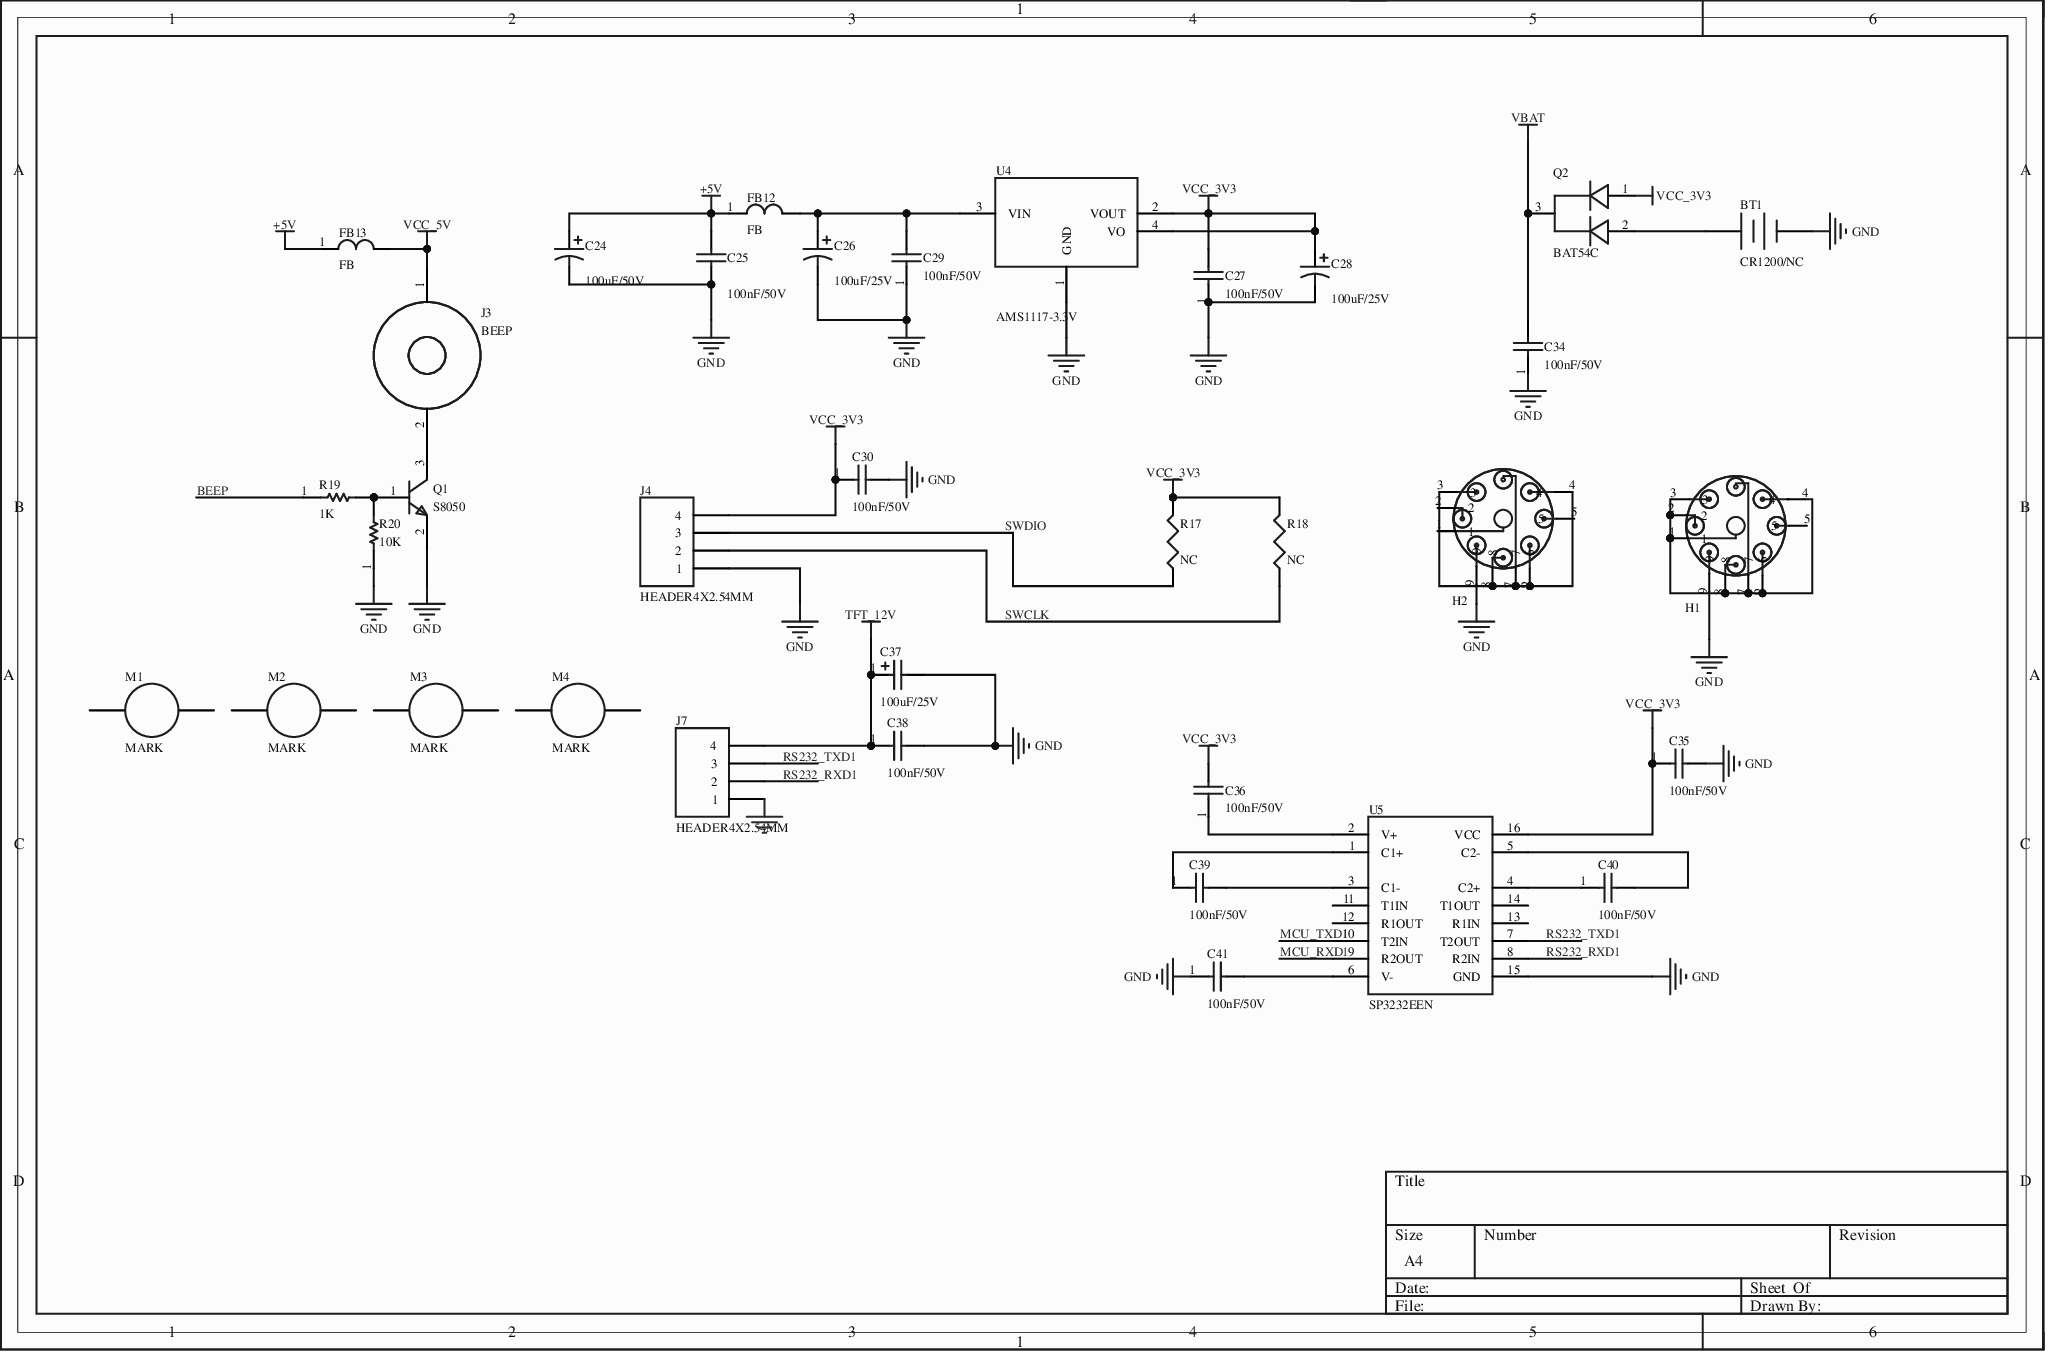
[diagram p0: MISC49890-3.schdoc]
# Altium project MISC49890-2.PrjPcb
1 sheet, 35 parts. Net scope: global (net labels, ports and power ports of the same name join across sheets).
Board file: MISC49890.pcbdoc

## Sheet MISC49890-3.schdoc
size 292 x 193 mm; @Page No: 1; @Page Count: 1; @Schematic Name: MISC49890; @Project Name: MISC49890; @Board Name: MISC49890; @Update Date: 2024-12-12; @Create Time: 18:15:27; @Update Time: 18:15:33; @Create Date: 2024-12-12

### Parts
BT1  CR1200/NC  [BAT-2]
C24  value 100uF/50V  [C0805]
C25  value 100nF/50V  [RAD-0.3]
C26  value 100uF/25V  [C0805]
C27  value 100nF/50V  [0603_C]  (hidden comment: Cap)
C28  value 100uF/25V  [C0805]
C29  value 100nF/50V  [0603_C]  (hidden comment: Cap)
C30  value 100nF/50V  [0603_C]  (hidden comment: Cap)
C34  value 100nF/50V  [0603_C]  (hidden comment: Cap)
C35  value 100nF/50V  [0603_C]  (hidden comment: Cap)
C36  value 100nF/50V  [0603_C]  (hidden comment: Cap)
C37  value 100uF/25V  [CAP-SMD_BD6.3-L6.6-W6.6-FD]  (hidden comment: Cap Pol1)
C38  value 100nF/50V  [0603_C]  (hidden comment: Cap)
C39  value 100nF/50V  [0603_C]  (hidden comment: Cap)
C40  value 100nF/50V  [0603_C]  (hidden comment: Cap)
C41  value 100nF/50V  [0603_C]  (hidden comment: Cap)
FB12  FB  [0603_L]
FB13  FB  [0603_L]
H1  H  [HOLE-ZR]  (value not drawn)
H2  H  [HOLE-ZR]  (value not drawn)
J3  BEEP  [BUZ-TH_BD12.0-P7.60-D0.6-FD]
J4  HEADER4X2.54MM  [CN4$2F$DIP$2F$P2.54B]
J7  HEADER4X2.54MM  [CN4$2F$DIP$2F$P2.54B]
M1  MARK  [RAD-0.1]
M2  MARK  [RAD-0.1]
M3  MARK  [RAD-0.1]
M4  MARK  [RAD-0.1]
Q1  S8050  [SOT-23(SOT-23-3)]
Q2  BAT54C  [SOT-23(SOT-23-3)]
R17  value NC  [J1-0603]
R18  value NC  [J1-0603]
R19  1K  [0603_R]
R20  10K  [0603_R]
U4  AMS1117-3.3V  [SOT-223]
U5  SP3232EEN  [SOP-16_150MIL]

### Nets
+5V: C24.1 C25.2 FB12.1 FB13.1
GND: BT1.2(-) C24.2 C25.1 C26.2 C27.1 C28.2 C29.1 C30.2 C34.1 C35.2 C37.2 C38.2 C41.1 H1.9 H2.9 J4.1 J7.1 Q1.2(E) R20.1 U4.1(GND) U5.15(GND)
TFT_12V: C37.1 C38.1 J7.4
VBAT: C34.2 Q2.3(K)
VCC_3V3: C27.2 C28.1 C30.1 C35.1 C36.2 J4.4 Q2.1(A1) R17.2 R18.2 U4.2(VOUT) U4.4(VO) U5.16(VCC)
VCC_5V: FB13.2 J3.1
BEEP: R19.1
MCU_RXD1: U5.9(R2OUT)
MCU_TXD1: U5.10(T2IN)
RS232_RXD1: J7.2 U5.8(R2IN)
RS232_TXD1: J7.3 U5.7(T2OUT)
SWCLK: J4.2 R18.1
SWDIO: J4.3 R17.1
NetBT1_1: BT1.1(+) Q2.2(A2)
NetC26_1: C26.1 C29.2 FB12.2 U4.3(VIN)
NetC36_1: C36.1 U5.2(V+)
NetC39_1: C39.1 U5.1(C1+)
NetC39_2: C39.2 U5.3(C1-)
NetC40_1: C40.1 U5.4(C2+)
NetC40_2: C40.2 U5.5(C2-)
NetC41_2: C41.2 U5.6(V-)
NetH1_1: H1.1 H1.2 H1.3 H1.4 H1.6 H1.7 H1.8
NetH2_3: H2.3 H2.4 H2.6 H2.7 H2.8
NetJ3_2: J3.2 Q1.3(C)
NetQ1_1: Q1.1(B) R19.2 R20.2

Not connected (* = marked no-connect by the designer): H1 5; H2 1 2 5; M1 1 2; M2 1 2; M3 1 2; M4 1 2; U5 11(T1IN)* 12(R1OUT)* 13(R1IN)* 14(T1OUT)*

### Notes on the sheet
- 1
- 2
- 3
- 4
- 5
- 6
- A
- B
- C
- D
- Title
- File:
- Date:
- Size
- A4
- Number
- Drawn By:
- Sheet
- Of
- Revision

### Library data of the parts
BT1 = CR1200/NC: Multicell Battery; AddInBom: yes; Origin Footprint: BAT-2; Device: CR1200/NC; Symbol: Battery; Design Item ID: Battery; Library Name: Miscellaneous Devices; Published: 24-Mar-1999; LatestRevisionDate: 17-Jul-2002; LatestRevisionNote: Re-released for DXP Platform.; PackageReference: BAT-2; FootprintName: BAT-2; ConvertToPcb: yes; Publisher: Altium Limited
C24 C26 C28 = Cap Pol3: Polarized Capacitor (Surface Mount); Origin Footprint 2: 1812; Origin Footprint 3: 1825; Origin Footprint 4: C2225; Origin Footprint 5: 2220; AddInBom: yes; Origin Footprint 1: C0805; Device: Cap Pol3; Symbol: Cap Pol3; Design Item ID: Cap Pol3; Library Name: Miscellaneous Devices; Published: 8-Jun-2000; LatestRevisionDate: 17-Jul-2002; LatestRevisionNote: Re-released for DXP Platform.; PackageReference: C0805; FootprintName: C0805; ConvertToPcb: yes; Publisher: Altium Limited
C25 = Cap: Capacitor; Origin Footprint 2: VP32-3.2; Origin Footprint 3: VP45-3.2; AddInBom: yes; Origin Footprint 1: RAD-0.3; Device: Cap; Symbol: Cap; Design Item ID: Cap; Library Name: Miscellaneous Devices; Published: 8-Jun-2000; LatestRevisionDate: 17-Jul-2002; LatestRevisionNote: Re-released for DXP Platform.; PackageReference: RAD-0.3; FootprintName: RAD-0.3; ConvertToPcb: yes; Publisher: Altium Limited
C27 C29 C30 C34-C36 C38-C41 = Cap: Capacitor; AddInBom: yes; Origin Footprint: 0603_C; Device: Cap; Symbol: Cap; Design Item ID: Cap; Library Name: UltraSonic; Published: 8-Jun-2000; LatestRevisionDate: 17-Jul-2002; LatestRevisionNote: Re-released for DXP Platform.; PackageReference: RAD-0.3; PackageDescription: Radial Cap, Thru-Hole; 2 Leads; 0.3 in Pin Spacing; FootprintName: 0603_C; ConvertToPcb: yes; Publisher: Altium Limited
C37 = Cap Pol1: Polarized Capacitor (Radial); AddInBom: yes; ModelId: ec7f1c7bda5e4386b54ec5ff3d1d94ff; Origin Footprint: CAP-SMD_BD6.3-L6.6-W6.6-FD; Device: Cap Pol1; Symbol: Cap Pol1; Design Item ID: Cap Pol1; Library Name: UltraSonic; Published: 8-Jun-2000; LatestRevisionDate: 17-Jul-2002; LatestRevisionNote: Re-released for DXP Platform.; PackageReference: RB7.6-15; PackageDescription: Polarized Capacitor (Radial); 2 Leads; FootprintName: CAP-SMD_BD6.3-L6.6-W6.6-FD; ConvertToPcb: yes; ModelName: CAP-SMD_BD6.3-L6.6-W6.6-FD; Publisher: Altium Limited
FB12 FB13 = FB: AddInBom: yes; Origin Footprint: 0603_L; Device: FB; Symbol: FB; Design Item ID: FB; Library Name: UltraSonic; FootprintName: 0603_L; ConvertToPcb: yes
H1 H2 = H: AddInBom: yes; Origin Footprint: HOLE-ZR; Device: H; Symbol: H; Design Item ID: H; Library Name: UltraSonic; FootprintName: HOLE-ZR; ConvertToPcb: yes
J3 = BEEP: AddInBom: yes; Origin Footprint: BUZ-TH_BD12.0-P7.60-D0.6-FD; Device: BEEP; Symbol: BEEP; Design Item ID: BEEP; Library Name: UltraSonic; FootprintName: BUZ-TH_BD12.0-P7.60-D0.6-FD; ConvertToPcb: yes
J4 J7 = HEADER4X2.54MM: Header, 4-Pin; AddInBom: yes; Origin Footprint: CN4$2F$DIP$2F$P2.54B; Device: HEADER4X2.54MM; Symbol: Header 4; Design Item ID: Header 4; Library Name: UltraSonic; LatestRevisionDate: 17-Jul-2002; LatestRevisionNote: Re-released for DXP Platform.; FootprintName: CN4$2F$DIP$2F$P2.54B; ConvertToPcb: yes; Publisher: Altium Limited
M1-M4 = MARK: Indicating Instrument; Symbol: Meter; Note: Place a &quot;letter&quot; into the symbol to show the function of the meter or instrument; AddInBom: yes; Origin Footprint: RAD-0.1; Device: MARK; Design Item ID: Meter; Library Name: Miscellaneous Devices; Published: 24-Mar-1999; LatestRevisionDate: 17-Jul-2002; LatestRevisionNote: Re-released for DXP Platform.; PackageReference: RAD-0.1; FootprintName: RAD-0.1; ConvertToPcb: yes; Publisher: Altium Limited
Q1 = S8050: NPN Bipolar Transistor; Symbol: QNPN; AddInBom: yes; Origin Footprint: SOT-23(SOT-23-3); Device: S8050; Design Item ID: QNPN; Library Name: UltraSonic; Published: 8-Jun-2000; LatestRevisionDate: 29-May-2009; LatestRevisionNote: IPC-7351 Footprint Added.; PackageVersion: Aug-1999; PackageReference: SOT-23B; PackageDescription: 3-Pin SOT-23 Package 0.95 mm Pitch, 2.4 mm Lead Span; FootprintName: SOT-23(SOT-23-3); ConvertToPcb: yes; Publisher: Altium Limited
Q2 = BAT54C: Manufacturer: CJ(江苏长电/长晶); Symbol: BAT54C_C2135; Add into BOM: yes; Forward Voltage (Vf@If): 1V@100mA; Reverse Voltage (Vr): 30V; Average Rectified Current (Io): 200mA; Origin Footprint: SOT-23(SOT-23-3); Device: BAT54C; Design Item ID: BAT54C_C2135; Library Name: UltraSonic; LCSC Part Name: 电压:30V 电流:200mA; Supplier Part: C2135; Manufacturer Part: BAT54C; Supplier Footprint: SOT-23; JLCPCB Part Class: Extended Part; Datasheet: https://atta.szlcsc.com/upload/public/pdf/source/20140809/1457707206468.pdf; Supplier: LCSC; Convert to PCB: yes; Diode Configuration: -; Reverse Leakage Current (Ir): -; FootprintName: SOT-23(SOT-23-3)
R17 R18 = Res3: Resistor; Origin Footprint 2: 3225[1210]; Origin Footprint 3: 5025[2010]; Origin Footprint 4: 6332[2512]; AddInBom: yes; Origin Footprint 1: J1-0603; Device: Res3; Symbol: Res3; Design Item ID: Res3; Library Name: Miscellaneous Devices; Published: 8-Jun-2000; LatestRevisionDate: 04-Mar-2005; LatestRevisionNote: PCB Footprint replaced.; PackageReference: J1-0603; FootprintName: J1-0603; ConvertToPcb: yes; Publisher: Altium Limited
R19 = 1K: Resistor; Symbol: Res1; Value: 100K; AddInBom: yes; ModelId: 7ef6e8be5b50432185c9142f7839acb7; Origin Footprint: 0603_R; Device: 1K; Design Item ID: Res1; Library Name: UltraSonic; Published: 8-Jun-2000; LatestRevisionDate: 17-Jul-2002; LatestRevisionNote: Re-released for DXP Platform.; PackageReference: AXIAL-0.3; PackageDescription: Axial Device, Thru-Hole; 2 Leads; 0.3 in Pin Spacing; FootprintName: 0603_R; ConvertToPcb: yes; ModelName: 0603_R; Publisher: Altium Limited
R20 = 10K: Resistor; Symbol: Res1; Value: 100K; AddInBom: yes; ModelId: 7ef6e8be5b50432185c9142f7839acb7; Origin Footprint: 0603_R; Device: 10K; Design Item ID: Res1; Library Name: UltraSonic; Published: 8-Jun-2000; LatestRevisionDate: 17-Jul-2002; LatestRevisionNote: Re-released for DXP Platform.; PackageReference: AXIAL-0.3; PackageDescription: Axial Device, Thru-Hole; 2 Leads; 0.3 in Pin Spacing; FootprintName: 0603_R; ConvertToPcb: yes; ModelName: 0603_R; Publisher: Altium Limited
U4 = AMS1117-3.3V: AddInBom: yes; Origin Footprint: SOT-223; Device: AMS1117-3.3V; Symbol: AMS1117-3.3V; Design Item ID: AMS1117-3.3V; Library Name: UltraSonic; FootprintName: SOT-223; ConvertToPcb: yes
U5 = SP3232EEN: AddInBom: yes; Origin Footprint: SOP-16_150MIL; Device: SP3232EEN; Symbol: SP3232EEN; Design Item ID: SP3232EEN; Library Name: UltraSonic; FootprintName: SOP-16_150MIL; ConvertToPcb: yes